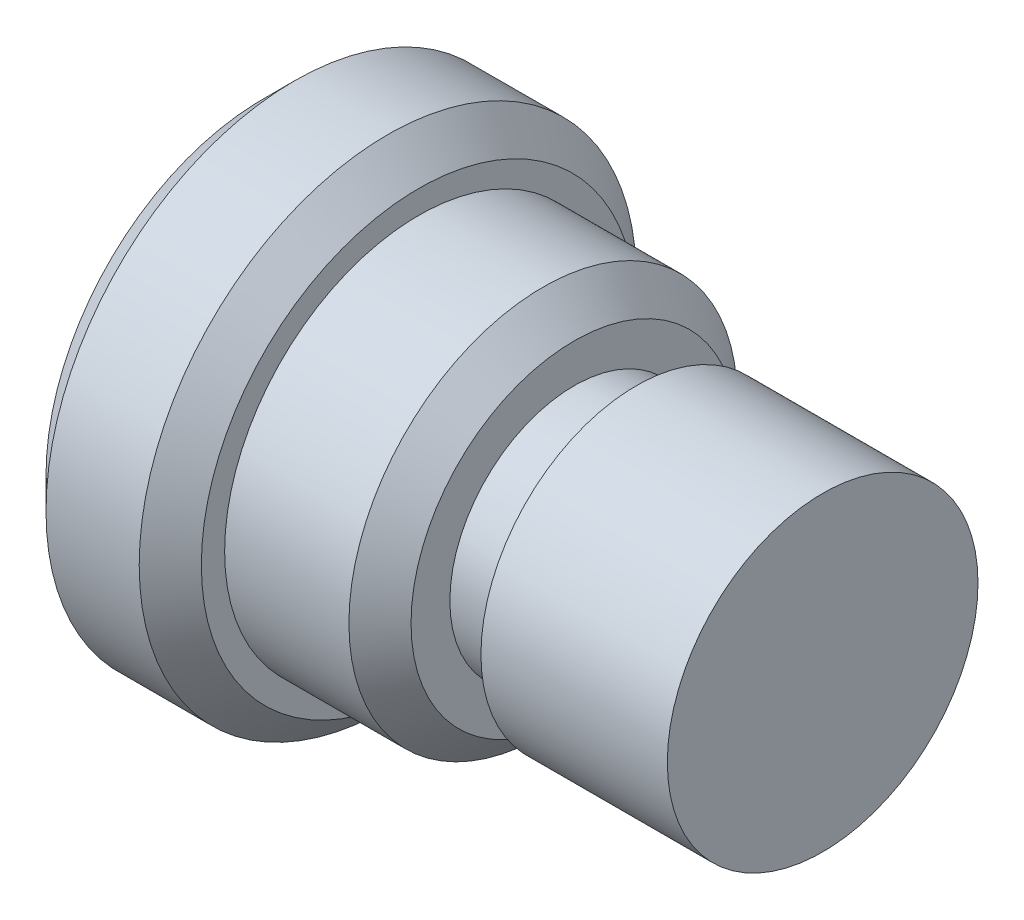
from build123d import *

# Parameters (mm, degrees)
CHAMFER_1_SIZE = 1


with BuildPart() as part:
    # 草图1 → 旋转1 (revolve)
    with BuildSketch(Plane.XY, mode=Mode.PRIVATE) as revolve_1_sk:
        Polygon((-116.444838016, -84.118352239), (-122.444838016, -84.118352239), (-122.444838016, -85.118352239), (-124.444838016, -85.118352239), (-124.444838016, -82.868352239), (-129.444838016, -82.868352239), (-129.444838016, -81.118352239), (-134.444838016, -81.118352239), (-134.444838016, -89.118352239), (-116.444838016, -89.118352239), align=None)
    revolve(revolve_1_sk.sketch.rotate(Axis((-129.444838016, -89.118352239, 0), (1, 0, 0)), 90), axis=Axis((-129.444838016, -89.118352239, 0), (1, 0, 0)))

    # 倒角1
    chamfer_1_edges = [part.edges().sort_by_distance(p)[0] for p in [
        (-124.444838016, -89.118352239, -6.25),
        (-134.444838016, -89.118352239, -8),
        (-129.444838016, -89.118352239, -8),
    ]]
    chamfer(chamfer_1_edges, length=CHAMFER_1_SIZE)


solid = part.part
